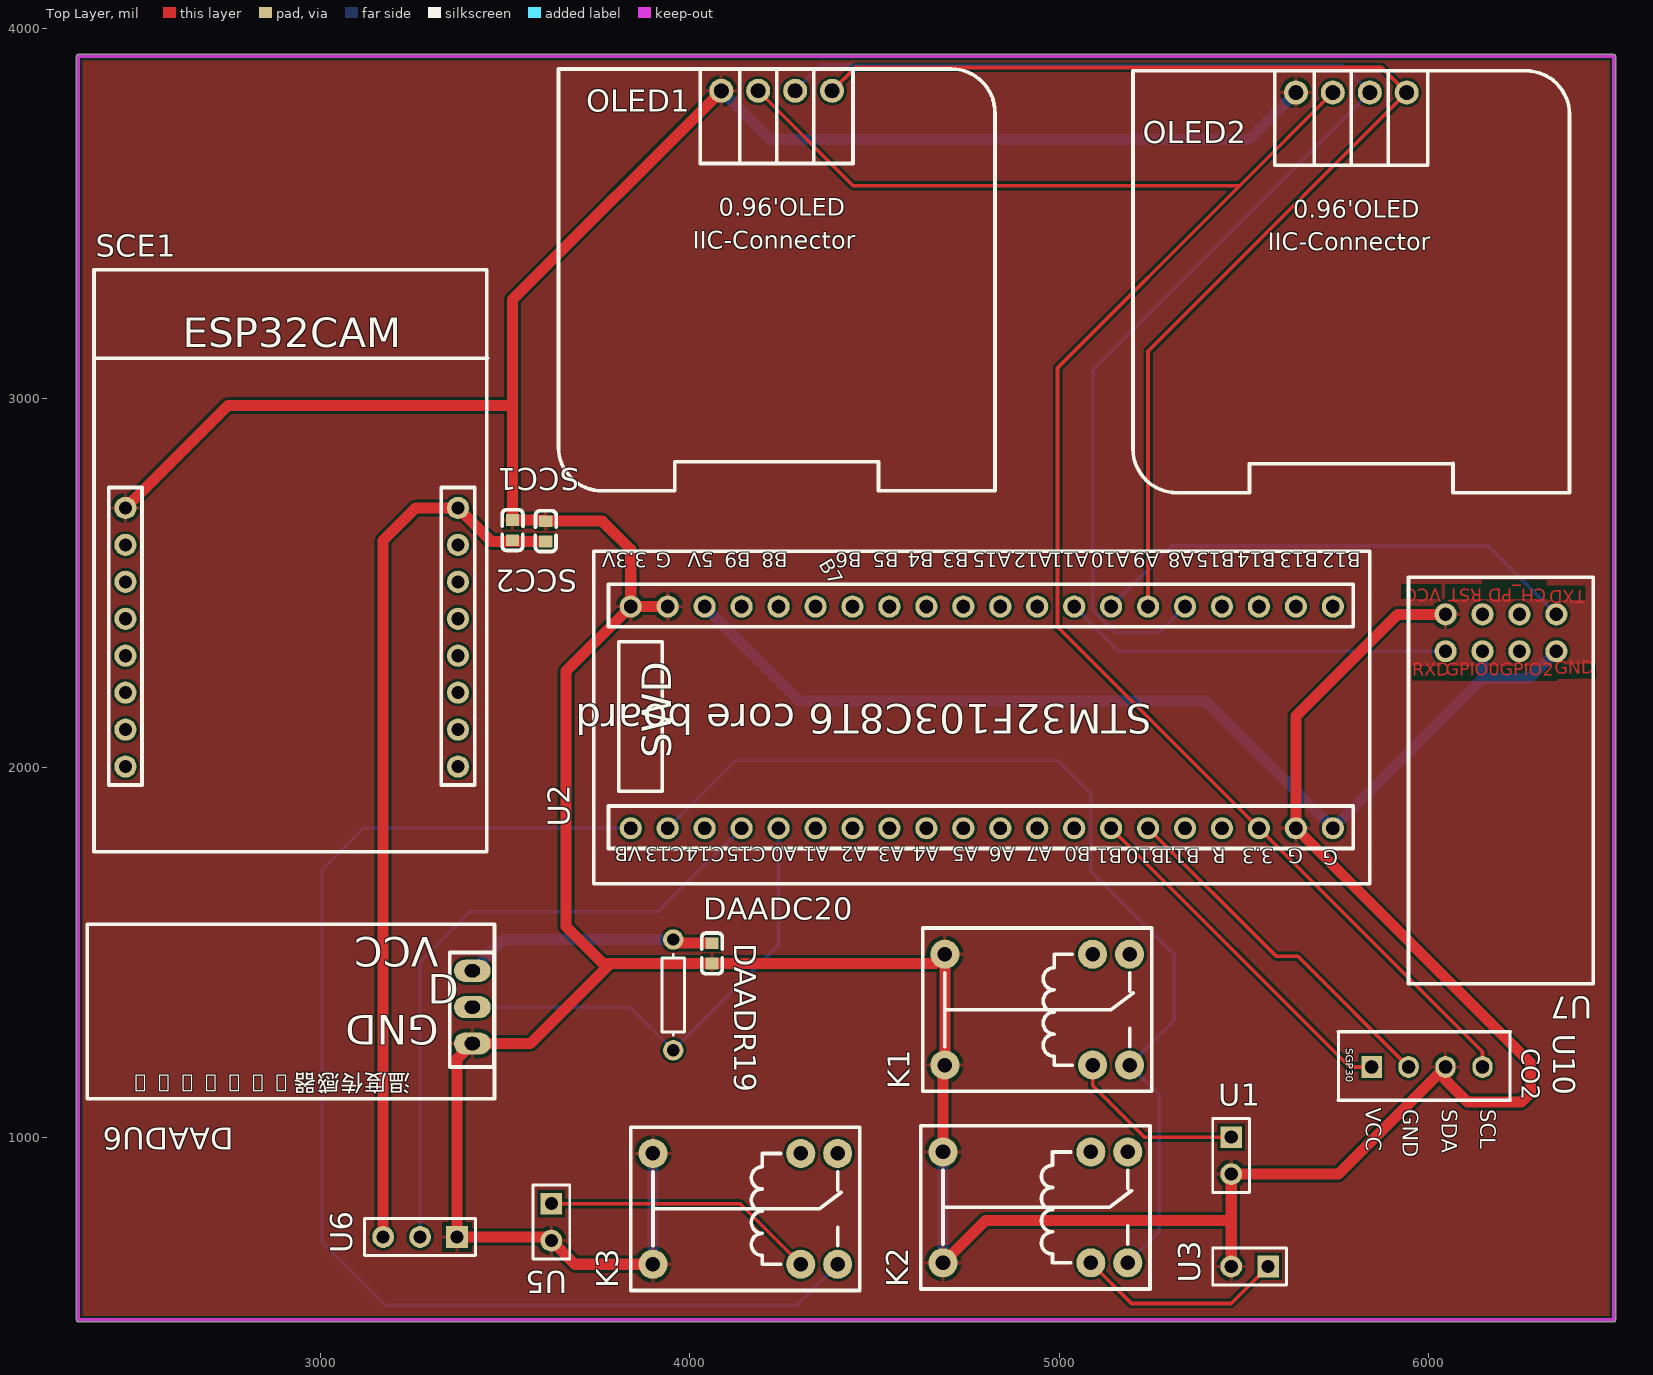
[diagram p0: Top Layer view]
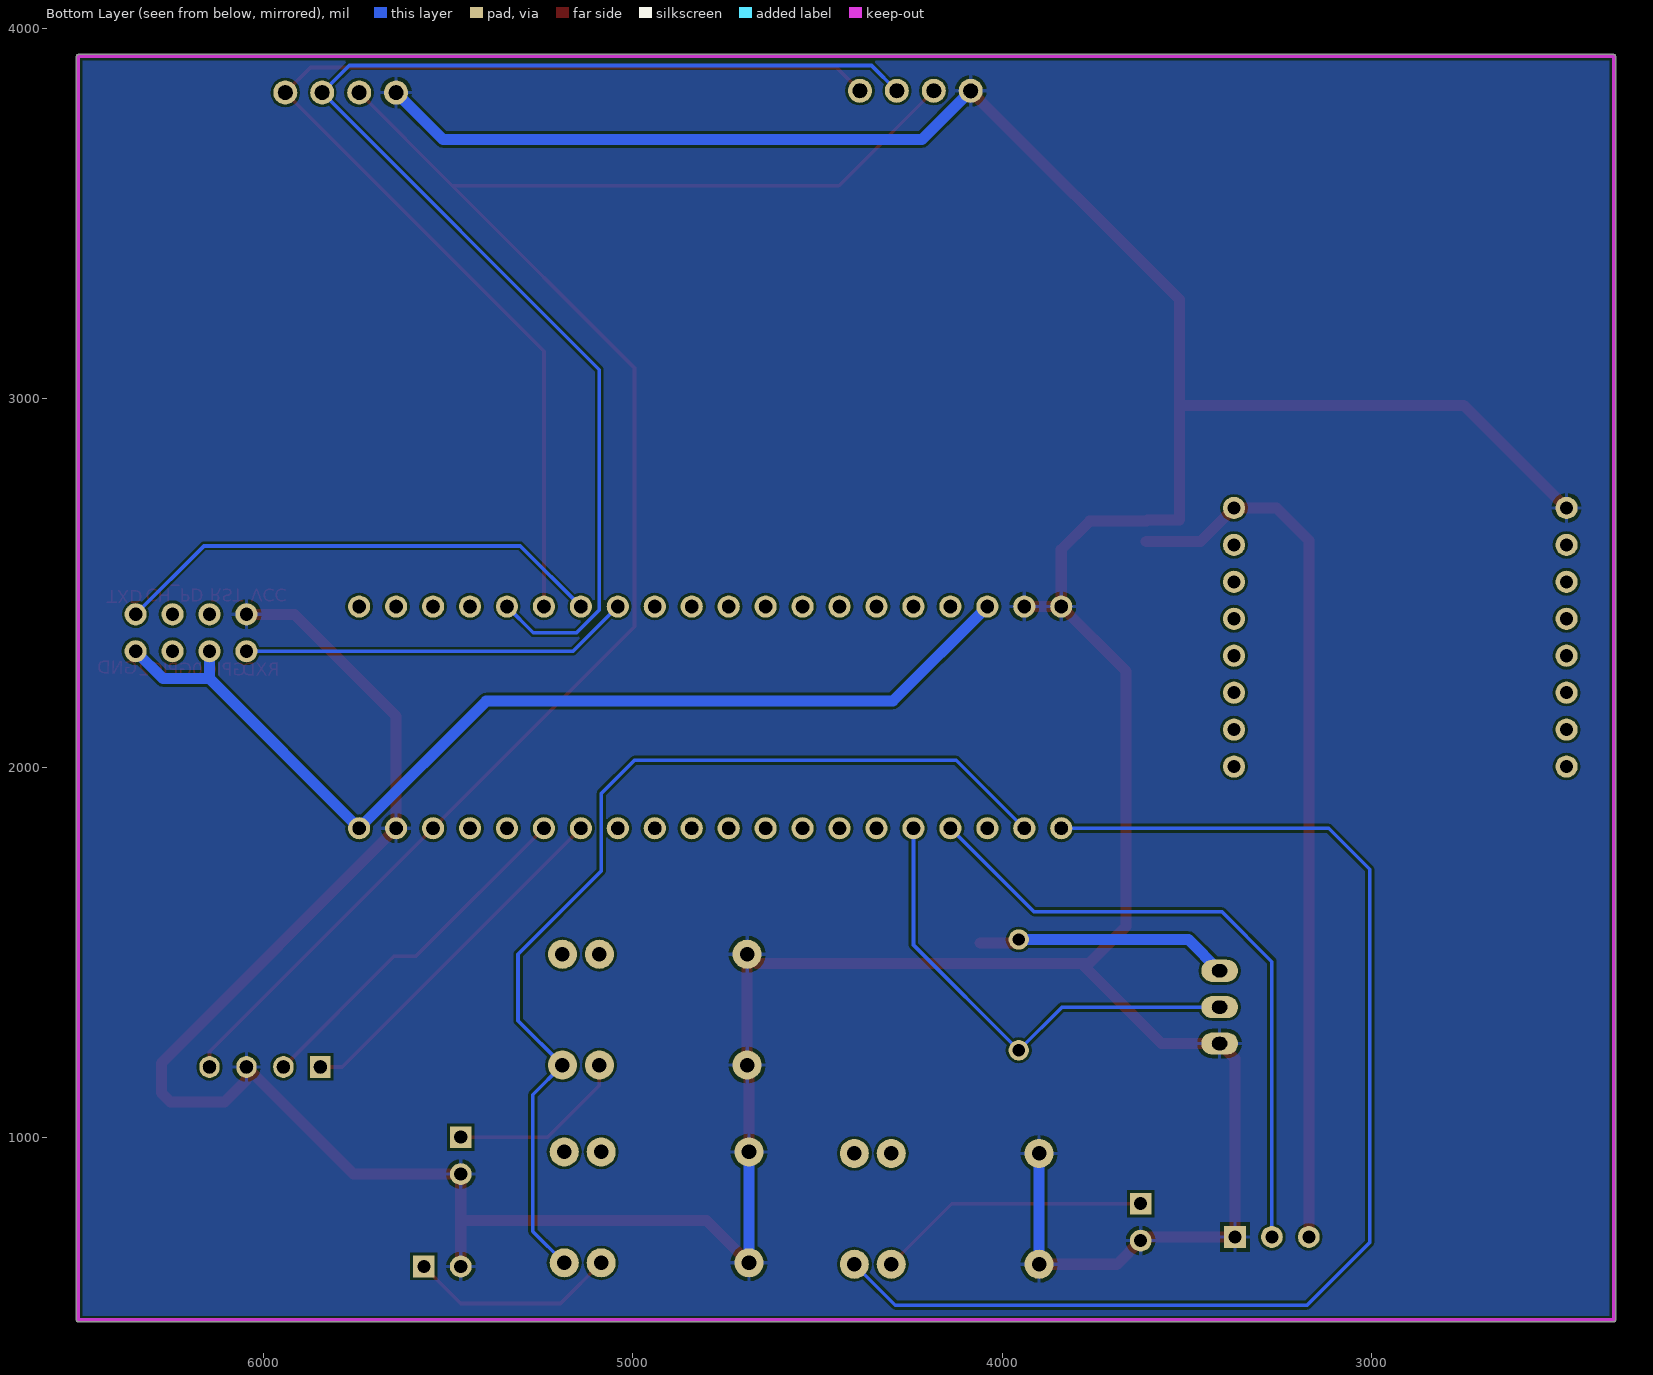
[diagram p1: Bottom Layer view, seen from below]
# Altium PCB MISC82816.PcbDoc
Units mil, origin at the board's own origin, x right, y up, seen from the top; angles counter-clockwise.
Board outline 4165.03 x 3430.03 mil, 2 copper layers (Top Layer, Bottom Layer); 18 components, 42 nets, 114 pads, 0 vias.

## Layer stack, top to bottom (the 12.6 mil dielectric is the usual default, probably not edited)
Top Solder: solder mask 0.4, Solder Resist, Dk 3.5
Top Layer: signal copper 1.4
Dielectric 1: dielectric 12.6, FR-4, Dk 4.8
Bottom Layer: signal copper 1.4
Bottom Solder: solder mask 0.4, Solder Resist, Dk 3.5

## Board outline
2339.99,505 ccw(c2345,505) 2345,499.99 6500,499.99 ccw(c6500,505) 6505.02,505 6505.02,3925 ccw(c6500,3925) 6500,3930.01 2345,3930.01 ccw(c2345,3925) 2339.99,3925

## Design rules (kind name [scope] priority, off if disabled: settings)
Clearance [All] p1: gap=7 ignorepadtopadclearanceinfootprint=FALSE except(0: Arc-Text Arc-Hole Track-Text Track-Hole SMDPad-Text SMDPad-Hole THPad-Text THPad-Hole Via-Text Via-Hole Fill-Text Fill-Hole Poly-Text Poly-Hole Region-Text Region-Hole Text-Text Text-Hole)
MinimumSolderMaskSliver [All] p1: minsoldermaskwidth=0
PolygonConnect [All] p1: connectstyle=Relief reliefconductorwidth=10 reliefentries=4 polygonreliefangle="90 Angle" airgapwidth=10
RoutingVias [All] p1: holewidth=28 width=50 viastyle="Through Hole" minholewidth=28 minwidth=50 maxholewidth=28 maxwidth=50
SilkToSilkClearance [All] p1: silktosilkclearance=0
SilkToSolderMaskClearance [IsPad] p1: minsilkscreentomaskgap=0 clearancetoexposedcopper=TRUE
SolderMaskExpansion [All] p1: expansion=4
Width [All] p1: maxlimit=30 minlimit=10 preferedwidth=10
27 further rules are at their usual default settings.

## Components (designator, comment, footprint, x,y, rotation, side; value= is the part's Value field where it differs from the comment)
DAADC20 "104" C0603 4059.89,1497.25 r90 top
DAADR19 "4.7k" AXIAL-0.3 3955,1385 r270 top
DAADU6 "DS18B20+" DS18B20 2920,1340 r180 top
K1 "HK4100F-DC3V-SHG relay" HK4100F 4940,1345 r180 top
K2 "HK4100F-DC3V-SHG relay" HK4100F 4935,810 r180 top
K3 "HK4100F-DC3V-SHG relay" HK4100F 4150,806 r180 top
OLED1 "0.96OLED_4P_MODULE_JX" 0.96OLED_4P 4235,3320 r0 top
OLED2 "0.96OLED_4P_MODULE_JX" 0.96OLED_4P 5790,3315 r0 top
SCC1 "0.1uF" C0603 3610,2640 r270 top
SCC2 "0.1u" C0603 3520.11,2642.86 r270 top
SCE1 "ESP32CAM" ESP32CAM 2920,2560 r0 top
U1 "DC motor terminal" HDR1X2 5465,1000 r270 top
U2 "STM32F103C8T6 system board" STM32核心板 4566,3337.5 r90 top
U3 "DC motor terminal" HDR1X2 5565,650 r180 top
U5 "DC motor terminal" hdr1x2 3625,820 r270 top
U6 "Turbidity module" HDR1X3 3370,730 r180 top
U7 "ESP-01S module" WIFI 6195,1965 r270 top
U10 "SGP30" SGP30 6024.57,1151.47 r270 top

## Footprints (in the part's own frame and the unit in brackets; to place one, negate y for a bottom-side part, rotate by r counter-clockwise, add the part's x,y. Pads: shape width x height; smd on the part's side, far side on the other; paste and mask are expansions set on the pad)
0.96OLED_4P [mm]
  round 1.65 hole 1 slot 1.005 at 0 deg paste+0 mask+0.051: 1(-3.811,12.997) 2(-1.271,13) 3(1.269,13) 4(3.809,13)
  silkscreen extent -15,-14.5 15,14.5
AXIAL-0.3 [mm] "Axial Device, Thru-Hole; 2 Leads; 0.3 in Pin Spacing"
  round 1.4 hole 0.85: 1(-3.81,0) 2(3.81,0)
  silkscreen extent -2.77,-0.76 2.77,0.76
C0603 [mm]
  rect 0.8x0.9 smd paste+0 mask+0.051: 1(-0.692,-0.003) 2(0.708,-0.003)
  silkscreen extent -1.4,-0.71 1.4,0.71
DS18B20 [mil]
  oval 99.37x60 hole 35.43 slot 41.34 at 0 deg paste+0 mask+4: 1(-491.35,86.55) 2(-491.35,-11.88) 3(-491.35,-110.3)
  silkscreen extent -551,-236 551,236
ESP32CAM [mil]
  round 60 hole 35.43 paste+0 mask+4: 1(452.5,-557.08) 2(452.5,-457.08) 3(452.5,-357.08) 4(452.5,-257.08) 5(452.5,-157.08) 6(452.5,-57.08) 7(452.5,42.92) 8(452.5,142.92) 9(-447.5,-557.08) 10(-447.5,-457.08) 11(-447.5,-357.08) 12(-447.5,-257.08) 13(-447.5,-157.08) 14(-447.5,-57.08) 15(-447.5,42.92) 16(-447.5,142.92)
  silkscreen extent -533,-787 533,787
HDR1X2 [mm] "Connector; Header; 2 Position"
  rect 1.5x1.5 hole 0.9: 1(0,0)
  round 1.5 hole 0.9: 2(2.54,0)
  silkscreen extent -1.27,-1.27 3.81,1.27
hdr1x2 [mm] "Connector; Header; 2 Position"
  rect 1.5x1.5 hole 0.9: 1(0,0)
  round 1.5 hole 0.9: 2(2.54,0)
  silkscreen extent -1.27,-1.27 3.81,1.27
HDR1X3 [mm] "Connector; Header; 3 Position"
  rect 1.5x1.5 hole 0.9: 1(0,0)
  round 1.5 hole 0.9: 2(2.54,0) 3(5.08,0)
  silkscreen extent -1.27,-1.27 6.35,1.27
HK4100F [mm] "单刀双投"
  round 2 hole 1: 1(-3.81,3.81) 2(-3.81,-3.81) 3(6.35,3.81) 3(6.35,-3.81) 4(-6.35,3.81) 5(-6.35,-3.81)
  silkscreen extent -7.87,-5.61 7.87,5.61, body extent -7.75,-5.5 7.75,5.5, height 12.2
SGP30 [mm]
  rect 1.5x1.4 hole 0.9 slot 0.905 at 0 deg paste+0 mask+0.051: 1(-0.979,-4.561)
  oval 1.5x1.4 hole 0.9 slot 0.905 at 0 deg paste+0 mask+0.051: 2(-0.979,-2.021) 3(-0.979,0.519) 4(-0.979,3.059)
  silkscreen extent -3.39,-6.85 1.31,4.96
STM32核心板 [mil]
  round 60 hole 36 slot 36.2 at 0 deg paste+0 mask+2: 1(-1501.5,726) 2(-1501.5,626) 3(-1501.5,526) 4(-1501.5,426) 5(-1501.5,326) 6(-1501.5,226) 7(-1501.5,126) 8(-1501.5,26) 9(-1501.5,-74) 10(-1501.5,-174) 11(-1501.5,-274) 12(-1501.5,-374) 13(-1501.5,-474) 14(-1501.5,-574) 15(-1501.5,-674) 16(-1501.5,-774) 17(-1501.5,-874) 18(-1501.5,-974) 19(-1501.5,-1074) 20(-1501.5,-1174) 21(-901.5,-1174) 22(-901.5,-1074) 23(-901.5,-974) 24(-901.5,-874) 25(-901.5,-774) 26(-901.5,-674) 27(-901.5,-574) 28(-901.5,-474) 29(-901.5,-374) 30(-901.5,-274) 31(-901.5,-174) 32(-901.5,-74) 33(-901.5,26) 34(-901.5,126) 35(-901.5,226) 36(-901.5,326) 37(-901.5,426) 38(-901.5,526) 39(-901.5,626) 40(-901.5,726)
  silkscreen extent -1652,-1274 -751,826
WIFI [mil]
  round 60 hole 36 paste+4 mask+2: 1(-350,150) 2(-350,50) 3(-350,-50) 4(-350,-150) 5(-450,-150) 6(-450,-50) 7(-450,50) 8(-450,150)
  silkscreen extent -550,-250 550,250

## Part data
K1 K2 K3: library part HK4100F-DC3V-SHG继电器
U1 U3 U5: library part 直流电机端子
U2: library part STM32F103C8T6系统板
U6: library part 浑浊度模块
U7: library part ESP-01S模块

## Nets (pads, with @x,y where several pads share a name; then routed paths per layer and width w, separated by ;. In a path a pad name is that pad's centre, name@x,y a point inside that pad or via, vN(x,y) a via of type N, cw(c..) or ccw(c..) an arc to the next point about the centre after c; other vN are vias at no path point)
3.3V: U2.20 U2.38 U7.1 U7.3 | length 2825.9
  Bottom Layer w30: U2.38 4296,2180 5396,2180 U2.20 6145,2241 ; U7.3 6145,2241 ; U7.1 6271,2241 6145,2241
5V: OLED1.2 OLED2.2 U2.18 U10.4 | length 4831.3
  Top Layer w10: OLED1.2 4441.75,3575 5488.14,3575 ; OLED2.2 5488.14,3575 ; U10.4 6145,1231 U2.18 4995,2381 4995,3081.86 5488.14,3575
GND: DAADC20.1 DAADU6.1 K1.3 K2.3 K3.3 OLED1.1 OLED2.1 SCC1.1 SCC2.1 SCE1.16 U1.2 U2.19 U2.39 U2.40 U3.2 U5.2 U6.1 U7.5 U10.3 | length 13423.9
  Top Layer w30: SCE1.16 2749.59,2980 3520,2980 ; K3.3@3900,656 3689,656 U5.2 3615,730 U6.1 3370,1212.1 DAADU6.1 3568.45,1253.45 3785,1470 ; U2.39 U2.40 ; OLED1.1 3520,3266.76 3520,2980 ; K2.3@4685,660 4800,775 5465,775 ; K2.3@4685,960 4685,1190 4690,1195 4690,1495 4665,1470 DAADC20.1 3785,1470 ; U3.2 5465,775 ; U7.5 5915,2415 5640,2140 U2.19 6275,1201 6275,1120 6250,1095 6105,1095 6045,1155 U10.3 5755,900 U1.2 5465,775 ; 3520,2980 SCC2.1 3607.03,2670.11 SCC1.1 3762.75,2667.25 3840,2590 U2.40 ; 3785,1470 3765,1470 3665,1570 3665,2261 U2.40
  Bottom Layer w30: K3.3@3900,656 K3.3@3900,956 ; OLED1.1 4216.65,3700 5513.24,3700 OLED2.1 ; K2.3@4685,660 K2.3@4685,960
NC: U2.37
NetK1_1: K1.1 U1.1 | length 488
  Top Layer w10: K1.1 5090,1140 5230,1000 U1.1
NetK2_1: K2.1 U3.1 | length 567
  Top Layer w10: K2.1 5195,550 5465,550 U3.1
NetK3_1: K3.1 U5.1 | length 742.9
  Top Layer w10: U5.1 4136,820 K3.1
PA0: OLED1.3 OLED2.3 U2.25 | length 3629.3
  Bottom Layer w10: OLED1.3 4353.14,3900 5766.75,3900 OLED2.3 5090,3076.86 5090,2426.6 5151.6,2365 5269,2365 U2.25
PA1: OLED1.4 OLED2.4 U2.26 | length 3290.2
  Top Layer w10: OLED1.4 4448.14,3895 5871.75,3895 OLED2.4 5240,3126.86 U2.26
PA2: U2.27 U7.8 | length 1349.6
  Bottom Layer w10: U2.27 5304,2600 6160,2600 U7.8
PA3: U2.28 U7.4 | length 1055.1
  Bottom Layer w10: U2.28 5161,2315 U7.4
PA4: U2.29
PA5: U2.30
PA6: U2.31
PA7: U2.32
PA8: DAADR19.2 DAADU6.2 U2.5 | length 1311.1
  Bottom Layer w10: DAADU6.2 3838.12,1351.88 DAADR19.2 4240,1520 U2.5
PA9: U2.6
PA10: U2.7
PA11: U2.8
PA12: U2.9
PA15: U2.10
PB0: U2.33
PB1: U2.34
PB3: U2.11
PB4: U2.12
PB5: U2.13
PB6: U2.14 U10.1 | length 972.6
  Top Layer w10: U2.14 5786,1190 U10.1
PB7: U2.15 U10.2 | length 972.6
  Top Layer w10: U2.15 5586,1490 5645,1490 U10.2
PB8: U2.16
PB9: U2.17
PB10: U2.35
PB11: U2.36
PB12: K3.4 U2.1 | length 3402.4
  Bottom Layer w10: U2.1 3116,1836 3005,1725 3005,715 3175,545 4289,545 K3.4
PB13: K1.4 K2.4 U2.2 | length 2739.7
  Bottom Layer w10: U2.2 4124,2020 4995,2020 5085,1930 5085,1720 5310,1495 5310,1315 K1.4 5270,1115 5270,745 K2.4
PB14: U2.3
PB15: U2.4 U6.2 | length 1764.5
  Bottom Layer w10: U6.2 3270,1475 3405,1610 3914,1610 U2.4
PC13: U2.22
PC14: U2.23
PC15: U2.24
VBAT: U2.21
VCC: SCC1.2 SCC2.2 SCE1.8 U6.3 | length 2398.9
  Top Layer w30: U6.3 3170,2615 3257.92,2702.92 SCE1.8 3463.28,2612.14 SCC1.2
VCC3.3: DAADC20.2 DAADR19.1 DAADU6.3 | length 687.8
  Top Layer w30: DAADR19.1 3964.89,1525.11 DAADC20.2
  Bottom Layer w30: DAADU6.3 3496.05,1535 DAADR19.1
pads on no net: K1.2 K1.5 K2.2 K2.5 K3.2 K3.5 SCE1.1 SCE1.2 SCE1.3 SCE1.4 SCE1.5 SCE1.6 SCE1.7 SCE1.9 SCE1.10 SCE1.11 SCE1.12 SCE1.13 SCE1.14 SCE1.15 U7.2 U7.6 U7.7

## Polygon pours and split planes (outlines as drawn)
GND on Bottom Layer "Top Layer-No Net" (solid, remove dead copper, pour order 18): 1710,4660 1860,4510 7025,4510 7025,230 6795,0 6375,420 2300,420
GND on Top Layer "Top Layer-No Net" (solid, remove dead copper, pour order 20): 2025,4165 7215,4165 6695,3645 6695,265 1240,265 1155,180

## Keep-outs
Keep-Out Layer:
  lines w10: 6500,1425 6500,3912.93 6500,3925 6450,3925 5950,3925 2345,3925 2345,505 6500,505 6500,1440